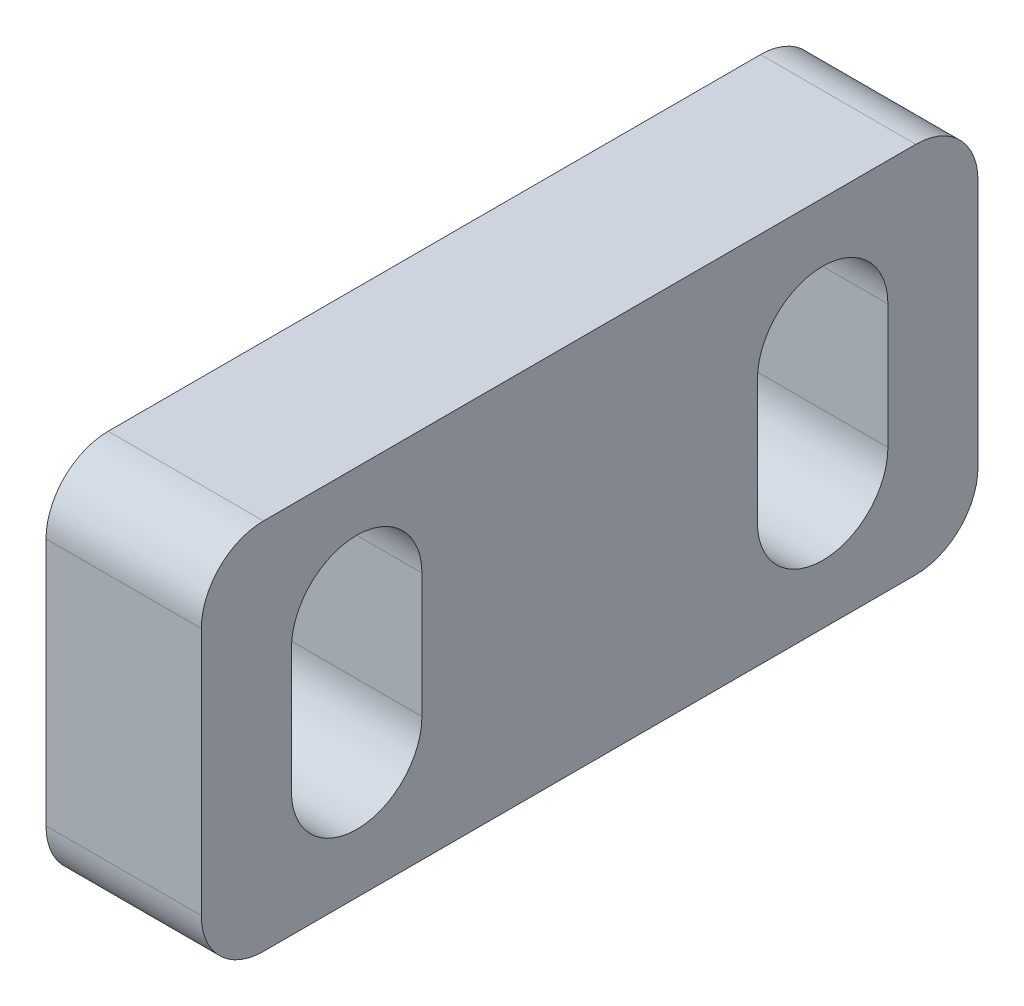
from build123d import *

# Parameters (mm, degrees)
EXTRUDE_1_DEPTH             = 5
EXTRUDE_2_DEPTH             = 5
FILLET_1_R                  = 2
CUT_EXTRUDE_1_DEPTH         = 13
FILLET_2_R                  = 2
HOLE_WIZARD_4_3_4_3_1_D     = 4.3
HOLE_WIZARD_4_3_4_3_1_DEPTH = 10.1
HOLE_WIZARD_4_3_4_3_1_TIP   = 1.291850331
SKETCH_7_W                  = 24.449376322
SKETCH_7_H                  = 27.885292322
CUT_EXTRUDE_2_DEPTH         = 10
CUT_EXTRUDE_3_DEPTH         = 10
FILLET_3_R                  = 5
SKETCH_9_W                  = 36.796643843
SKETCH_9_H                  = 32.156214513
CUT_EXTRUDE_4_DEPTH         = 21
FILLET_4_R                  = 2


with BuildPart() as part:
    # 草图1 → 凸台-拉伸1 (new body)
    with BuildSketch(Plane(origin=(0, 0, 0), x_dir=(0, 0, -1), z_dir=(1, 0, 0))):
        Polygon((-12.5, 6), (-6, 6), (-6, 61), (6, 61), (6, 6), (12.5, 6), (12.5, -6), (-12.5, -6), align=None)
    extrude(amount=EXTRUDE_1_DEPTH)

    # 草图2 → 凸台-拉伸2 (add)
    with BuildSketch(Plane.ZY):
        Polygon((-6, 61), (-12.5, 6), (12.5, 6), (6, 61), align=None)
    extrude(amount=-EXTRUDE_2_DEPTH)

    # 圆角1
    fillet_1_edges = [part.edges().sort_by_distance(p)[0] for p in [
        (2.5, 61, 6),
        (2.5, 61, -6),
    ]]
    fillet(fillet_1_edges, radius=FILLET_1_R)

    # 草图3 → 切除-拉伸1 (cut)
    with BuildSketch(Plane.ZY):
        with BuildLine():
            Line((-5.4, 2), (-5.4, -2))
            ThreePointArc((-5.4, -2), (-7.5, -4.1), (-9.6, -2))
            Line((-9.6, -2), (-9.6, 2))
            ThreePointArc((-9.6, 2), (-7.5, 4.1), (-5.4, 2))
        make_face()
        with BuildLine():
            Line((5.4, 2), (5.4, -2))
            ThreePointArc((5.4, -2), (7.5, -4.1), (9.6, -2))
            Line((9.6, -2), (9.6, 2))
            ThreePointArc((9.6, 2), (7.5, 4.1), (5.4, 2))
        make_face()
    extrude(amount=-CUT_EXTRUDE_1_DEPTH, mode=Mode.SUBTRACT)

    # 圆角2
    fillet_2_edges = [part.edges().sort_by_distance(p)[0] for p in [
        (2.5, -6, -12.5),
        (2.5, -6, 12.5),
    ]]
    fillet(fillet_2_edges, radius=FILLET_2_R)

    # Ø4.3 (4.3) 直径孔1
    with Locations(Plane.ZY):
        with Locations((0, 56), (0, 41)):
            Hole(HOLE_WIZARD_4_3_4_3_1_D / 2, depth=HOLE_WIZARD_4_3_4_3_1_DEPTH)
            with Locations((0, 0, -(HOLE_WIZARD_4_3_4_3_1_DEPTH + HOLE_WIZARD_4_3_4_3_1_TIP / 2))):  # 118° drill point
                Cone(0, HOLE_WIZARD_4_3_4_3_1_D / 2, HOLE_WIZARD_4_3_4_3_1_TIP, mode=Mode.SUBTRACT)

    # 草图7 → 切除-拉伸2 (cut)
    with BuildSketch(Plane(origin=(5, 0, 0), x_dir=(0, 0, -1), z_dir=(1, 0, 0))):
        with Locations((-1.251346032, 49.942646161)):
            Rectangle(SKETCH_7_W, SKETCH_7_H)
    extrude(amount=-CUT_EXTRUDE_2_DEPTH, mode=Mode.SUBTRACT)

    # 草图8 → 切除-拉伸3 (cut)
    with BuildSketch(Plane.ZY):
        with BuildLine():
            Line((-1, 33.75), (1, 33.75))
            ThreePointArc((1, 33.75), (3.25, 31.5), (1, 29.25))
            Line((1, 29.25), (-1, 29.25))
            ThreePointArc((-1, 29.25), (-3.25, 31.5), (-1, 33.75))
        make_face()
    extrude(amount=-CUT_EXTRUDE_3_DEPTH, mode=Mode.SUBTRACT)

    # 圆角3
    fillet_3_edges = [part.edges().sort_by_distance(p)[0] for p in [
        (2.5, 36, 8.954545455),
        (2.5, 36, -8.954545455),
    ]]
    fillet(fillet_3_edges, radius=FILLET_3_R)

    # 草图9 → 切除-拉伸4 (cut)
    with BuildSketch(Plane(origin=(5, 0, 0), x_dir=(0, 0, -1), z_dir=(1, 0, 0))):
        with Locations((-3.006475341, 22.078107257)):
            Rectangle(SKETCH_9_W, SKETCH_9_H)
    extrude(amount=-CUT_EXTRUDE_4_DEPTH, mode=Mode.SUBTRACT)

    # 圆角4
    fillet_4_edges = [part.edges().sort_by_distance(p)[0] for p in [
        (2.5, 6, 12.5),
        (2.5, 6, -12.5),
    ]]
    fillet(fillet_4_edges, radius=FILLET_4_R)


solid = part.part
